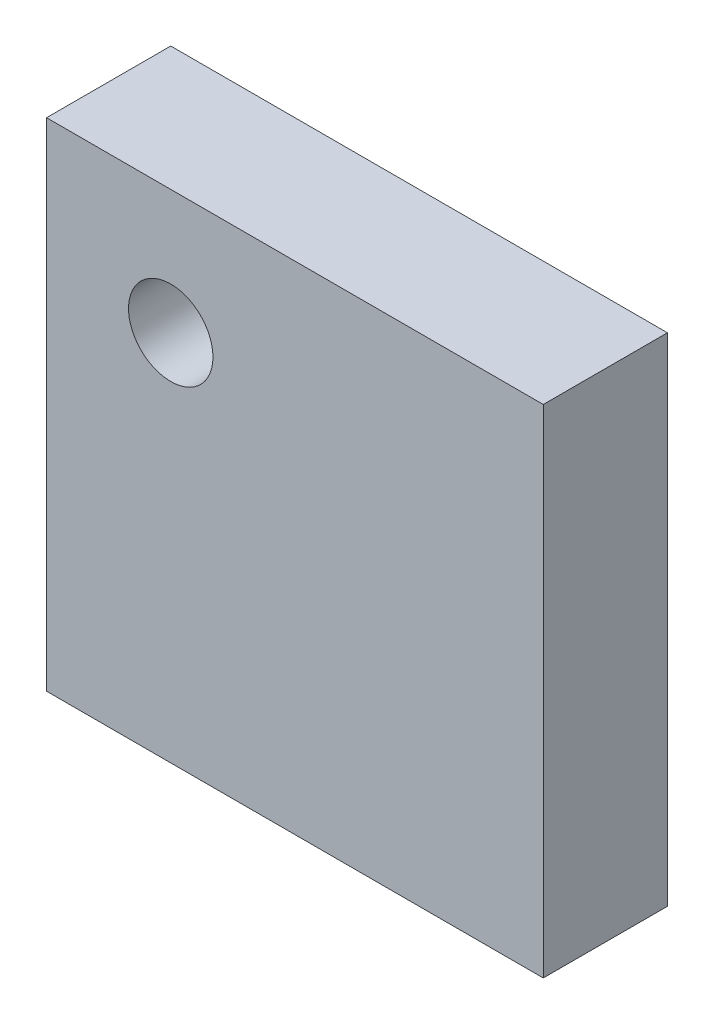
SolidWorks part; units mm, degrees
ref_plane "前视基准面" through (0, 0, 0) normal (0, 0, 1) x (1, 0, 0)
ref_plane "上视基准面" through (0, 0, 0) normal (0, 1, 0) x (1, 0, 0)
ref_plane "右视基准面" through (0, 0, 0) normal (1, 0, 0) x (0, 0, -1)
sketch "草图1" plane through (0, 0, 0) normal (0, 0, 1) x (1, 0, 0)
  line L1 (-20, -20) -> (20, -20)
  line L2 (-20, -20) -> (-20, 20)
  line L3 (-20, 20) -> (20, 20)
  line L4 (20, -20) -> (20, 20)
  line L5 (-20, -20) -> (20, 20) construction
  line L6 (-20, 20) -> (20, -20) construction
  point P0 (0, 0)
  dimension "D1" = 40
  dimension "D2" = 40
extrude "凸台-拉伸1" add sketch "草图1" along normal mid plane 10
hole_wizard "M8 螺纹孔1" positions "草图2" profile "草图3" tap size "M8" standard "GB" end condition through all
sketch "草图2" plane through (0, 0, 5) normal (0, 0, 1) x (1, 0, 0)
  line L0 (-20, 20) -> (-20, -20) construction
  line L1 (-20, -20) -> (20, -20) construction
  point P0 (-10, 10)
  dimension "D1" = 10
  dimension "D2" = 30
sketch "草图3" plane through (-10, 10, 5) normal (1, 0, 0) x (0, -1, 0)
  line L0 (0, 0) -> (0, 10)
  line L1 (0, 10) -> (3.4, 10)
  line L2 (3.4, 10) -> (3.4, 0)
  line L5 (3.4, 0) -> (0, 0)
  line L11 (0, -6.35) -> (0, 107.95) construction
  dimension "通孔螺纹孔钻头直径" = 6.8
  dimension "通孔螺纹孔钻头深度" = 10
cosmetic thread "孔螺蚊线1"
